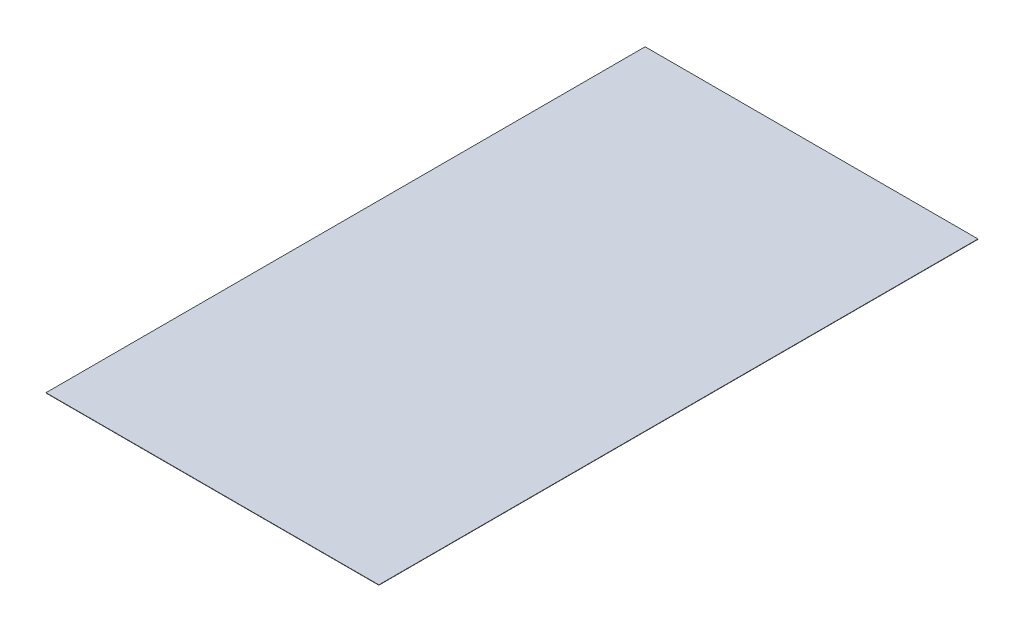
from build123d import *

# Parameters (mm, degrees)
SKETCH1_W           = 1000
SKETCH1_H           = 1800
BOSS_EXTRUDE1_DEPTH = 1


with BuildPart() as part:
    # Sketch1 → Boss-Extrude1 (new body)
    with BuildSketch(Plane(origin=(0, 0, 0), x_dir=(1, 0, 0), z_dir=(0, 1, 0))):
        Rectangle(SKETCH1_W, SKETCH1_H)
    extrude(amount=BOSS_EXTRUDE1_DEPTH)


solid = part.part
